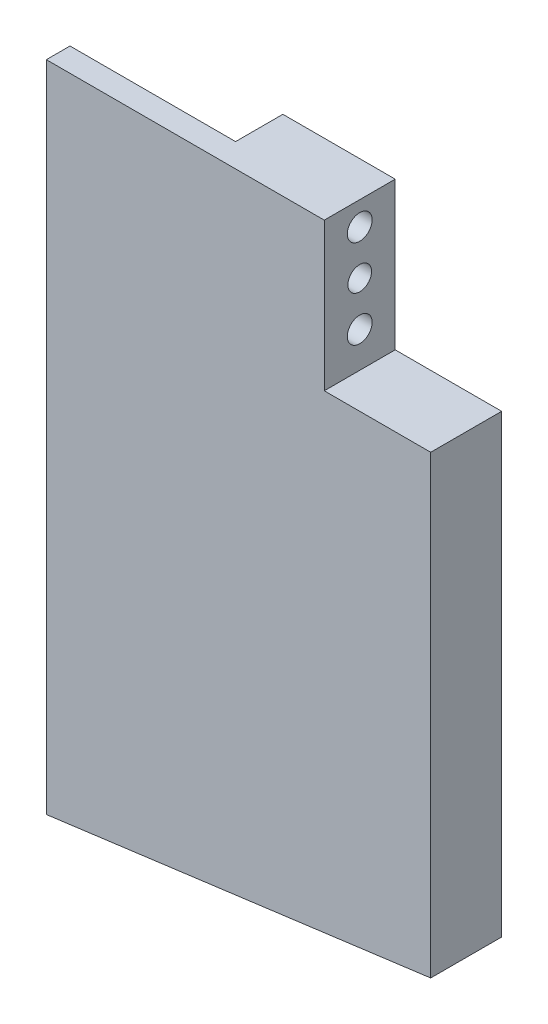
from build123d import *

# Parameters (mm, degrees)
SKETCH1_W                    = 65
SKETCH1_H                    = 12
BOSS_EXTRUDE1_DEPTH          = 51
BOSS_EXTRUDE2_DEPTH          = 12
SKETCH3_W                    = 18
SKETCH3_H                    = 25
CUT_EXTRUDE2_DEPTH           = 69.900909755
M5_TAPPED_HOLE1_D            = 4.2
M5_TAPPED_HOLE1_DEPTH        = 12.4
M5_TAPPED_HOLE1_TIP          = 1.2618073
M5_TAPPED_HOLE2_D            = 4.2
M5_TAPPED_HOLE2_DEPTH        = 12.4
M5_TAPPED_HOLE2_TIP          = 1.2618073
M5_TAPPED_HOLE3_D            = 4.2
M5_TAPPED_HOLE3_DEPTH        = 12.4
M5_TAPPED_HOLE3_TIP          = 1.2618073
CUT_EXTRUDE3_DEPTH           = 28
F_4_0_4_DIAMETER_HOLE1_D     = 4
F_4_0_4_DIAMETER_HOLE1_DEPTH = 8
F_4_0_4_DIAMETER_HOLE1_TIP   = 1.201721238


with BuildPart() as part:
    # Sketch1 → Boss-Extrude1 (new, symmetric)
    with BuildSketch(Plane(origin=(0, 0, 0), x_dir=(1, 0, 0), z_dir=(0, 1, 0))):
        Rectangle(SKETCH1_W, SKETCH1_H)
    extrude(amount=BOSS_EXTRUDE1_DEPTH, both=True)

    # Sketch4 → Boss-Extrude2 (add)
    with BuildSketch(Plane.XY.offset(6)):
        Polygon((-32.5, -51), (32.5, -51), (-32.5, -59.557412343), align=None)
    extrude(amount=-BOSS_EXTRUDE2_DEPTH)

    # Sketch3 → Cut-Extrude2 (cut, through all)
    with BuildSketch(Plane.XY.offset(6)):
        with Locations((23.5, 38.5)):
            Rectangle(SKETCH3_W, SKETCH3_H)
    extrude(amount=-CUT_EXTRUDE2_DEPTH, mode=Mode.SUBTRACT)

    # M5 Tapped Hole1
    with Locations(Plane(origin=(7.153590973, -54.336918053, 0), x_dir=(-0.9914448613738113, -0.13052619222004513, 0), z_dir=(0.13052619222004513, -0.9914448613738113, 0))):
        with Locations((-18.065122191, 0), (6.934877809, 0), (31.934877809, 0)):
            Hole(M5_TAPPED_HOLE1_D / 2, depth=M5_TAPPED_HOLE1_DEPTH)
            with Locations((0, 0, -(M5_TAPPED_HOLE1_DEPTH + M5_TAPPED_HOLE1_TIP / 2))):  # 118° drill point
                Cone(0, M5_TAPPED_HOLE1_D / 2, M5_TAPPED_HOLE1_TIP, mode=Mode.SUBTRACT)

    # M5 Tapped Hole2
    with Locations(Plane.ZY.offset(32.5)):
        with Locations((0, 43), (0, 3), (0, -37)):
            Hole(M5_TAPPED_HOLE2_D / 2, depth=M5_TAPPED_HOLE2_DEPTH)
            with Locations((0, 0, -(M5_TAPPED_HOLE2_DEPTH + M5_TAPPED_HOLE2_TIP / 2))):  # 118° drill point
                Cone(0, M5_TAPPED_HOLE2_D / 2, M5_TAPPED_HOLE2_TIP, mode=Mode.SUBTRACT)

    # M5 Tapped Hole3
    with Locations(Plane(origin=(14.5, 0, 0), x_dir=(0, 0, -1), z_dir=(1, 0, 0))):
        with Locations((0, 47), (0, 32)):
            Hole(M5_TAPPED_HOLE3_D / 2, depth=M5_TAPPED_HOLE3_DEPTH)
            with Locations((0, 0, -(M5_TAPPED_HOLE3_DEPTH + M5_TAPPED_HOLE3_TIP / 2))):  # 118° drill point
                Cone(0, M5_TAPPED_HOLE3_D / 2, M5_TAPPED_HOLE3_TIP, mode=Mode.SUBTRACT)

    # Sketch12 → Cut-Extrude3 (cut)
    with BuildSketch(Plane.ZY.offset(32.5)):
        Polygon((-6, 43), (-6, 51), (2, 51), align=None)
    extrude(amount=-CUT_EXTRUDE3_DEPTH, mode=Mode.SUBTRACT)

    # Ø4.0 (4) Diameter Hole1
    with Locations(Plane(origin=(14.5, 0, 0), x_dir=(0, 0, -1), z_dir=(1, 0, 0))):
        with Locations((0, 39.5)):
            Hole(F_4_0_4_DIAMETER_HOLE1_D / 2, depth=F_4_0_4_DIAMETER_HOLE1_DEPTH)
            with Locations((0, 0, -(F_4_0_4_DIAMETER_HOLE1_DEPTH + F_4_0_4_DIAMETER_HOLE1_TIP / 2))):  # 118° drill point
                Cone(0, F_4_0_4_DIAMETER_HOLE1_D / 2, F_4_0_4_DIAMETER_HOLE1_TIP, mode=Mode.SUBTRACT)


solid = part.part
